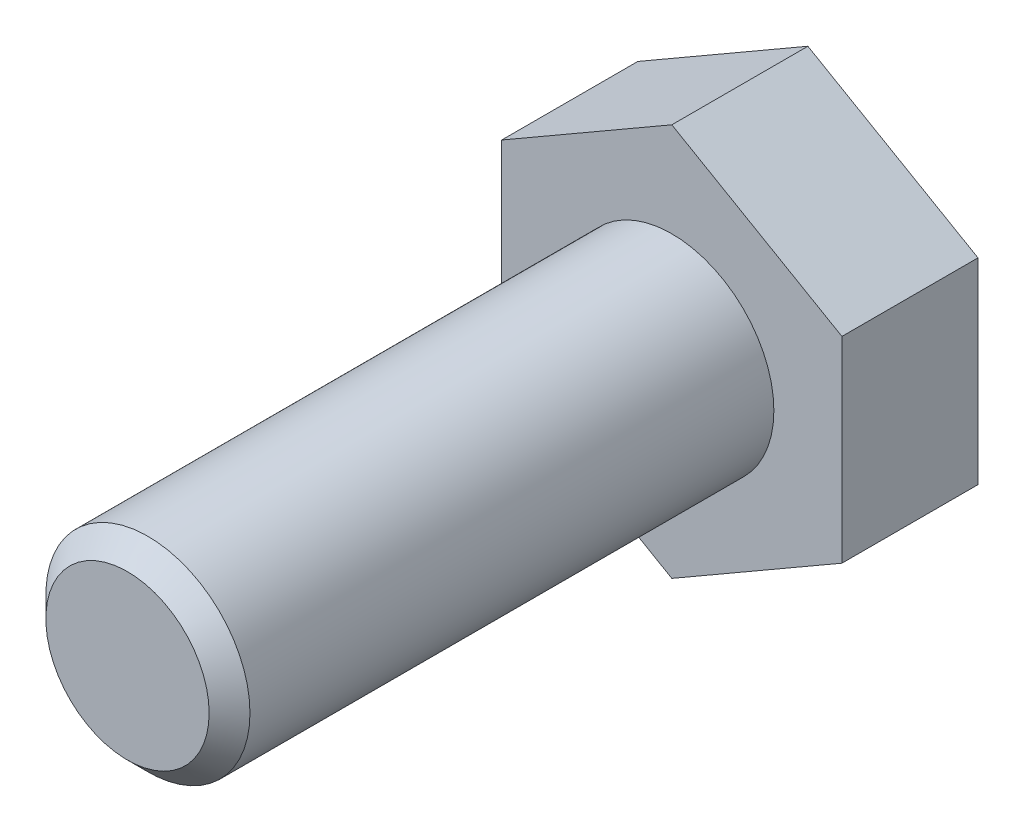
from build123d import *

# Parameters (mm, degrees)
BOSS_EXTRUDE1_DEPTH = 4
SKETCH3_R           = 3
BOSS_EXTRUDE2_DEPTH = 16
CHAMFER1_SIZE       = 0.6


with BuildPart() as part:
    # Sketch1 → Boss-Extrude1 (new body)
    with BuildSketch(Plane.XY):
        Polygon((5, 2.886751346), (0, 5.773502692), (-5, 2.886751346), (-5, -2.886751346), (0, -5.773502692), (5, -2.886751346), align=None)
    extrude(amount=BOSS_EXTRUDE1_DEPTH)

    # Sketch3 → Boss-Extrude2 (add)
    with BuildSketch(Plane.XY.offset(4)):
        Circle(SKETCH3_R)
    extrude(amount=BOSS_EXTRUDE2_DEPTH)

    # Chamfer1
    chamfer1_edges = [part.edges().sort_by_distance(p)[0] for p in [
        (-3, 0, 20),
    ]]
    chamfer(chamfer1_edges, length=CHAMFER1_SIZE)


solid = part.part
